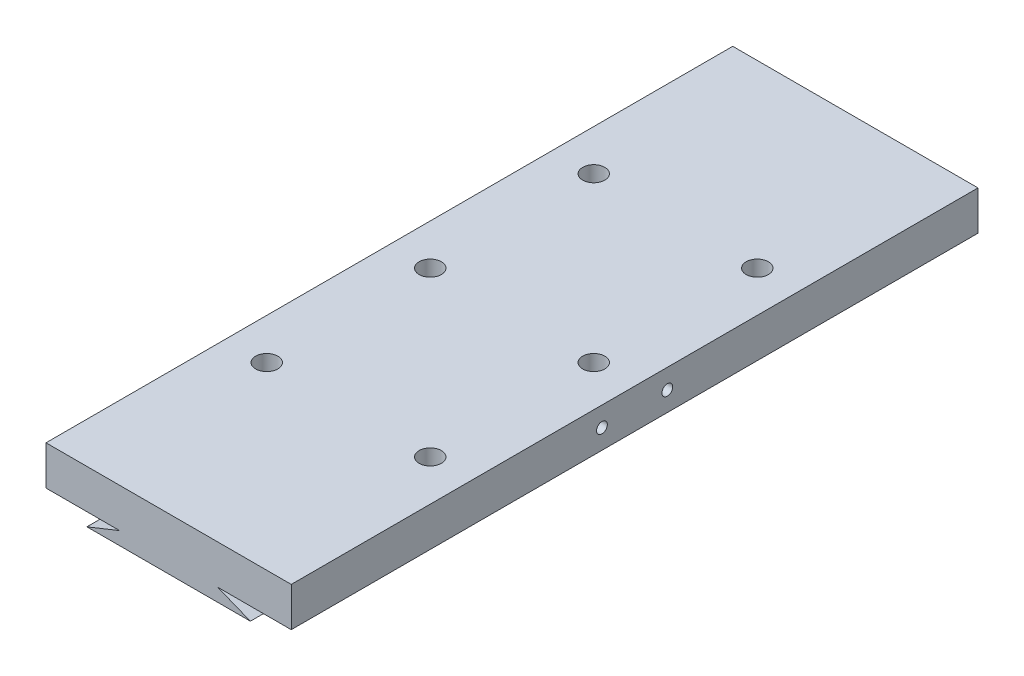
SolidWorks part; units mm, degrees
ref_plane "前视基准面" through (0, 0, 0) normal (0, 0, 1) x (1, 0, 0)
ref_plane "上视基准面" through (0, 0, 0) normal (0, 1, 0) x (1, 0, 0)
ref_plane "右视基准面" through (0, 0, 0) normal (1, 0, 0) x (0, 0, -1)
sketch "草图1" plane through (0, 0, 0) normal (0, 0, 1) x (1, 0, 0)
  line L0 (-25, -10) -> (25, -10)
  line L1 (-37.5, 6) -> (37.5, 6)
  line L2 (-37.5, 6) -> (-37.5, -6)
  line L3 (-37.5, -6) -> (-15, -6)
  line L4 (37.5, 6) -> (37.5, -6)
  line L5 (-37.5, 6) -> (37.5, -6) construction
  line L6 (-37.5, -6) -> (37.5, 6) construction
  line L7 (-15, -6) -> (-25, -10)
  line L8 (25, -10) -> (15, -6)
  line L9 (15, -6) -> (37.5, -6)
  point P0 (0, 0)
  dimension "D1" = 75
  dimension "D2" = 12
  dimension "D3" = 50
  dimension "D4" = 25
  dimension "D5" = 4
  dimension "D6" = 15
  dimension "D7" = 15
extrude "凸台-拉伸1" add sketch "草图1" along normal mid plane 210
hole_wizard "M4 螺纹孔1" positions "草图3" profile "草图2" tap size "M4" standard "ISO"
sketch "草图3" plane through (-37.5, 0, 0) normal (-1, 0, 0) x (0, 0, 1)
  point P0 (-10, 0)
  point P2 (10, 0)
  dimension "D1" = 10
  dimension "D2" = 20
sketch "草图2" plane through (-37.5, 0, -10) normal (0, 1, 0) x (0, 0, 1)
  line L0 (0, 0) -> (0, 11.0914)
  line L1 (0, 11.0914) -> (1.65, 10.1)
  line L2 (1.65, 10.1) -> (1.65, 0)
  line L5 (1.65, 0) -> (0, 0)
  line L10 (0, 11.0914) -> (-1.65, 10.1) construction
  line L11 (0, -6.35) -> (0, 107.95) construction
  dimension "螺纹孔钻头直径" = 3.3
  dimension "螺纹孔钻头深度" = 10.1
  dimension "导头角度" = 118
cosmetic thread "孔螺蚊线1" parameters "D1"=8, "D2"=4
cosmetic thread "孔螺蚊线2" parameters "D1"=8, "D2"=4
mirror "镜向1" about plane through (0, 0, 0) normal (1, 0, 0) of "M4 螺纹孔1"
hole_wizard "M8 螺纹孔1" positions "草图5" profile "草图4" tap size "M8" standard "ISO"
sketch "草图5" plane through (0, 6, 0) normal (0, 1, 0) x (1, 0, 0)
  point P0 (-25, 50)
  dimension "D1" = 25
  dimension "D2" = 50
sketch "草图4" plane through (-25, 6, -50) normal (1, 0, 0) x (0, 0, 1)
  line L0 (0, 0) -> (0, 21.7929)
  line L1 (0, 21.7929) -> (3.4, 19.75)
  line L2 (3.4, 19.75) -> (3.4, 0)
  line L5 (3.4, 0) -> (0, 0)
  line L10 (0, 21.7929) -> (-3.4, 19.75) construction
  line L11 (0, -6.35) -> (0, 107.95) construction
  dimension "螺纹孔钻头直径" = 6.8
  dimension "螺纹孔钻头深度" = 19.75
  dimension "导头角度" = 118
cosmetic thread "孔螺蚊线3" parameters "D1"=16, "D2"=8
pattern_linear "阵列(线性)1" count 3 spacing 50 along (0, 0, 1) count 2 spacing 50 along (1, 0, 0) of "M8 螺纹孔1"
